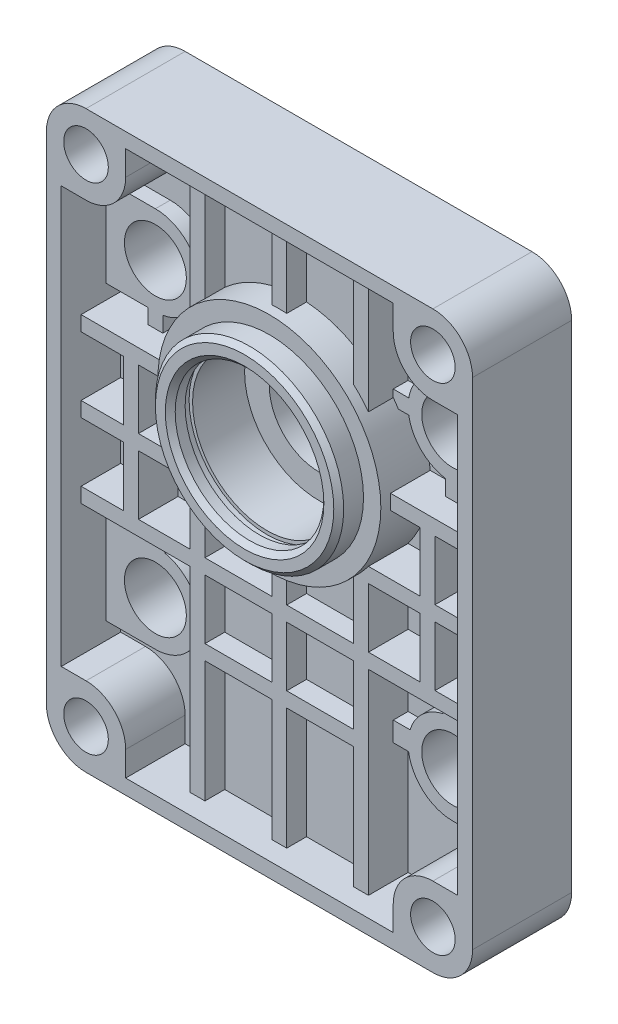
from build123d import *
from build123d.topology import SkipClean

# Parameters (mm, degrees)
EXTRUDE_1_DEPTH     = 12
SKETCH_2_R          = 22.5
EXTRUDE_2_DEPTH     = 6
SKETCH_3_R          = 19
EXTRUDE_3_DEPTH     = 5
EXTRUDE_4_DEPTH     = 8
SKETCH_5_W          = 10.424096596
SKETCH_5_H          = 12
SKETCH_5_W_2        = 13.5
EXTRUDE_5_DEPTH     = 4
CUT_EXTRUDE_START   = -4
SKETCH_6_W          = 8.575903404
SKETCH_6_H          = 12
SKETCH_6_W_2        = 10.424096596
CUT_EXTRUDE_1_DEPTH = 4
EXTRUDE_6_DEPTH     = 3
SKETCH_8_R          = 6.25
CUT_EXTRUDE_2_DEPTH = 87.423376467
SKETCH_9_R          = 4.5
CUT_EXTRUDE_3_DEPTH = 88.891979156
SKETCH_10_R         = 4
CUT_EXTRUDE_4_DEPTH = 6
CHAMFER_1_SIZE      = 1


with BuildPart() as part:
    # 草图1 → 凸台-拉伸1 (new body)
    with BuildSketch(Plane.XY):
        with BuildLine():
            Line((-43, 34), (-43, -66))
            ThreePointArc((-43, -66), (-40.656854249, -71.656854249), (-35, -74))
            Line((-35, -74), (35, -74))
            ThreePointArc((35, -74), (40.656854249, -71.656854249), (43, -66))
            Line((43, -66), (43, 34))
            ThreePointArc((43, 34), (40.656854249, 39.656854249), (35, 42))
            Line((35, 42), (-35, 42))
            ThreePointArc((-35, 42), (-40.656854249, 39.656854249), (-43, 34))
        make_face()
    extrude(amount=EXTRUDE_1_DEPTH)

    # 草图2 → 凸台-拉伸2 (add)
    with BuildSketch(Plane.XY.offset(12)):
        Circle(SKETCH_2_R)
    extrude(amount=EXTRUDE_2_DEPTH)

    # 草图3 → 凸台-拉伸3 (add)
    with BuildSketch(Plane.XY.offset(18)):
        Circle(SKETCH_3_R)
    extrude(amount=EXTRUDE_3_DEPTH)

    # 草图4 → 凸台-拉伸4 (add)
    with BuildSketch(Plane.XY.offset(12)):
        with BuildLine():
            Line((43, -66), (43, 34))
            ThreePointArc((43, 34), (40.656854249, 39.656854249), (35, 42))
            Line((35, 42), (-35, 42))
            ThreePointArc((-35, 42), (-40.656854249, 39.656854249), (-43, 34))
            Line((-43, 34), (-43, -66))
            ThreePointArc((-43, -66), (-40.656854249, -71.656854249), (-35, -74))
            Line((-35, -74), (35, -74))
            ThreePointArc((35, -74), (40.656854249, -71.656854249), (43, -66))
        make_face()
        with BuildLine():
            Line((35, -58), (40, -58))
            Line((40, -58), (40, 26))
            Line((40, 26), (35, 26))
            ThreePointArc((35, 26), (29.343145751, 28.343145751), (27, 34))
            Line((27, 34), (27, 39))
            Line((27, 39), (-27, 39))
            Line((-27, 39), (-27, 34))
            ThreePointArc((-27, 34), (-29.343145751, 28.343145751), (-35, 26))
            Line((-35, 26), (-40, 26))
            Line((-40, 26), (-40, -58))
            Line((-40, -58), (-35, -58))
            ThreePointArc((-35, -58), (-29.343145751, -60.343145751), (-27, -66))
            Line((-27, -66), (-27, -71))
            Line((-27, -71), (27, -71))
            Line((27, -71), (27, -66))
            ThreePointArc((27, -66), (29.343145751, -60.343145751), (35, -58))
        make_face(mode=Mode.SUBTRACT)
    extrude(amount=EXTRUDE_4_DEPTH)

    # 草图5 → 凸台-拉伸5 (add)
    # profile 1 of 3: a face of its own
    with BuildSketch(Plane.XY.offset(12)):
        with BuildLine():
            Line((-15, 16.770509831), (-15, 39))
            Line((-15, 39), (-18, 39))
            Line((-18, 39), (-18, 13.5))
            ThreePointArc((-18, 13.5), (-16.580834075, 15.209403057), (-15, 16.770509831))
        make_face()
    # profile 2 of 3: a face of its own
    with BuildSketch(Plane.XY.offset(12)):
        with BuildLine():
            Line((0, -71), (0, -22.5))
            ThreePointArc((0, -22.5), (-0.750417479, -22.487482598), (-1.5, -22.449944321))
            Line((-1.5, -22.449944321), (-1.5, -28.5))
            Line((-1.5, -28.5), (-15, -28.5))
            Line((-15, -28.5), (-15, -16.770509831))
            ThreePointArc((-15, -16.770509831), (-16.580834075, -15.209403057), (-18, -13.5))
            Line((-18, -13.5), (-28.424096596, -13.5))
            Line((-28.424096596, -13.5), (-28.424096596, -1.5))
            Line((-28.424096596, -1.5), (-22.449944321, -1.5))
            ThreePointArc((-22.449944321, -1.5), (-22.5, 0), (-22.449944321, 1.5))
            Line((-22.449944321, 1.5), (-40, 1.5))
            Line((-40, 1.5), (-40, -1.5))
            Line((-40, -1.5), (-31.424096596, -1.5))
            Line((-31.424096596, -1.5), (-31.424096596, -13.5))
            Line((-31.424096596, -13.5), (-40, -13.5))
            Line((-40, -13.5), (-40, -16.5))
            Line((-40, -16.5), (-31.424096596, -16.5))
            Line((-31.424096596, -16.5), (-31.424096596, -28.5))
            Line((-31.424096596, -28.5), (-40, -28.5))
            Line((-40, -28.5), (-40, -31.5))
            Line((-40, -31.5), (-18, -31.5))
            Line((-18, -31.5), (-18, -71))
            Line((-18, -71), (-15, -71))
            Line((-15, -71), (-15, -46.5))
            Line((-15, -46.5), (-1.5, -46.5))
            Line((-1.5, -46.5), (-1.5, -71))
            Line((-1.5, -71), (0, -71))
        make_face()
        with Locations((-23.212048298, -22.5)):
            Rectangle(SKETCH_5_W, SKETCH_5_H, mode=Mode.SUBTRACT)
        with Locations((-8.25, -37.5)):
            Rectangle(SKETCH_5_W_2, SKETCH_5_H, mode=Mode.SUBTRACT)
    # profile 3 of 3: a face of its own
    with BuildSketch(Plane.XY.offset(12)):
        with BuildLine():
            Line((0, 22.5), (0, 39))
            Line((0, 39), (-1.5, 39))
            Line((-1.5, 39), (-1.5, 22.449944321))
            ThreePointArc((-1.5, 22.449944321), (-0.750417479, 22.487482598), (0, 22.5))
        make_face()
    extrude_5 = extrude(amount=EXTRUDE_5_DEPTH)

    # 镜向1: 凸台-拉伸5 across plane
    add(extrude_5.mirror(Plane(origin=(0, 0, 0), x_dir=(0, 0, 1), z_dir=(1, 0, 0))))

    # 草图6 → 切除-拉伸1 (cut)
    with SkipClean():  # the faces are left unmerged after this step: merging them gives an invalid solid
        with BuildSketch(Plane.XY.offset(12).offset(CUT_EXTRUDE_START)):
            with Locations((-35.712048298, -7.5)):
                Rectangle(SKETCH_6_W, SKETCH_6_H)
            with BuildLine():
                Line((-28.424096596, -1.5), (-28.424096596, -13.5))
                Line((-28.424096596, -13.5), (-18, -13.5))
                ThreePointArc((-18, -13.5), (-21.096196313, -7.823074914), (-22.449944321, -1.5))
                Line((-22.449944321, -1.5), (-28.424096596, -1.5))
            make_face()
            with Locations((-35.712048298, -22.5)):
                Rectangle(SKETCH_6_W, SKETCH_6_H)
            with Locations((-23.212048298, -22.5)):
                Rectangle(SKETCH_6_W_2, SKETCH_6_H)
            with Locations((35.712048298, -7.5)):
                Rectangle(SKETCH_6_W, SKETCH_6_H)
            with Locations((35.712048298, -22.5)):
                Rectangle(SKETCH_6_W, SKETCH_6_H)
            with Locations((23.212048298, -22.5)):
                Rectangle(SKETCH_6_W_2, SKETCH_6_H)
            with BuildLine():
                Line((28.424096596, -1.5), (28.424096596, -13.5))
                Line((28.424096596, -13.5), (18, -13.5))
                ThreePointArc((18, -13.5), (21.096196313, -7.823074914), (22.449944321, -1.5))
                Line((22.449944321, -1.5), (28.424096596, -1.5))
            make_face()
            with BuildLine():
                Line((-40, 26), (-40, 1.5))
                Line((-40, 1.5), (-22.449944321, 1.5))
                ThreePointArc((-22.449944321, 1.5), (-21.096196313, 7.823074914), (-18, 13.5))
                Line((-18, 13.5), (-18, 39))
                Line((-18, 39), (-27, 39))
                Line((-27, 39), (-27, 34))
                ThreePointArc((-27, 34), (-29.343145751, 28.343145751), (-35, 26))
                Line((-35, 26), (-40, 26))
            make_face()
            with BuildLine():
                Line((18, 13.5), (18, 39))
                Line((18, 39), (27, 39))
                Line((27, 39), (27, 34))
                ThreePointArc((27, 34), (29.343145751, 28.343145751), (35, 26))
                Line((35, 26), (40, 26))
                Line((40, 26), (40, 1.5))
                Line((40, 1.5), (22.449944321, 1.5))
                ThreePointArc((22.449944321, 1.5), (21.096196313, 7.823074914), (18, 13.5))
            make_face()
            with BuildLine():
                Line((-40, -58), (-40, -31.5))
                Line((-40, -31.5), (-18, -31.5))
                Line((-18, -31.5), (-18, -71))
                Line((-18, -71), (-27, -71))
                Line((-27, -71), (-27, -66))
                ThreePointArc((-27, -66), (-29.343145751, -60.343145751), (-35, -58))
                Line((-35, -58), (-40, -58))
            make_face()
            with BuildLine():
                Line((40, -58), (40, -31.5))
                Line((40, -31.5), (18, -31.5))
                Line((18, -31.5), (18, -71))
                Line((18, -71), (27, -71))
                Line((27, -71), (27, -66))
                ThreePointArc((27, -66), (29.343145751, -60.343145751), (35, -58))
                Line((35, -58), (40, -58))
            make_face()
        extrude(amount=CUT_EXTRUDE_1_DEPTH, mode=Mode.SUBTRACT)

    # 草图7 → 凸台-拉伸6 (add)
    with SkipClean():  # the faces are left unmerged after this step: merging them gives an invalid solid
        with BuildSketch(Plane.XY.offset(8)):
            with BuildLine():
                Line((-30, 22.5), (-40, 22.5))
                Line((-40, 22.5), (-40, 4.5))
                Line((-40, 4.5), (-31.5, 4.5))
                Line((-31.5, 4.5), (-31.5, 1.5))
                Line((-31.5, 1.5), (-28.5, 1.5))
                Line((-28.5, 1.5), (-28.5, 4.625880325))
                ThreePointArc((-28.5, 4.625880325), (-23.636038969, 7.136038969), (-21.125880325, 12))
                Line((-21.125880325, 12), (-18, 12))
                Line((-18, 12), (-18, 15))
                Line((-18, 15), (-21.125880325, 15))
                ThreePointArc((-21.125880325, 15), (-24.190524981, 20.373863542), (-30, 22.5))
            make_face()
            with BuildLine():
                Line((-31.5, -31.5), (-28.023620394, -31.5))
                Line((-28.023620394, -31.5), (-28.023620394, -36.719685447))
                ThreePointArc((-28.023620394, -36.719685447), (-23.881575765, -38.899629944), (-21.394428301, -42.864827192))
                Line((-21.394428301, -42.864827192), (-18, -42.864827192))
                Line((-18, -42.864827192), (-18, -46.817586404))
                Line((-18, -46.817586404), (-21.096968715, -46.817586404))
                ThreePointArc((-21.096968715, -46.817586404), (-24.120300928, -52.313893074), (-30, -54.5))
                Line((-30, -54.5), (-40, -54.5))
                Line((-40, -54.5), (-40, -36.5))
                Line((-40, -36.5), (-31.5, -36.5))
                Line((-31.5, -36.5), (-31.5, -31.5))
            make_face()
        extrude_6 = extrude(amount=EXTRUDE_6_DEPTH)

    # 镜向2: 凸台-拉伸6 across plane
    with SkipClean():  # the faces are left unmerged after this step: merging them gives an invalid solid
        add(extrude_6.mirror(Plane(origin=(0, 0, 0), x_dir=(0, 0, 1), z_dir=(1, 0, 0))))

    # 草图8 → 切除-拉伸2 (cut, through all)
    with SkipClean():  # the faces are left unmerged after this step: merging them gives an invalid solid
        with BuildSketch(Plane.XY.offset(11)):
            with Locations((-30, 13.5)):
                Circle(SKETCH_8_R)
            with Locations((30, 13.5)):
                Circle(SKETCH_8_R)
            with Locations((-30, -45.5)):
                Circle(SKETCH_8_R)
            with Locations((30, -45.5)):
                Circle(SKETCH_8_R)
        extrude(amount=-CUT_EXTRUDE_2_DEPTH, mode=Mode.SUBTRACT)

    # 草图9 → 切除-拉伸3 (cut, through all)
    with SkipClean():  # the faces are left unmerged after this step: merging them gives an invalid solid
        with BuildSketch(Plane.XY.offset(20)):
            with Locations((-35, 34)):
                Circle(SKETCH_9_R)
            with Locations((35, 34)):
                Circle(SKETCH_9_R)
            with Locations((-35, -66)):
                Circle(SKETCH_9_R)
            with Locations((35, -66)):
                Circle(SKETCH_9_R)
        extrude(amount=-CUT_EXTRUDE_3_DEPTH, mode=Mode.SUBTRACT)

    # 草图10 → 切除-拉伸4 (cut)
    with SkipClean():  # the faces are left unmerged after this step: merging them gives an invalid solid
        with BuildSketch(Plane(origin=(0, 0, 0), x_dir=(-1, 0, 0), z_dir=(0, 0, -1))):
            with Locations((0, 31)):
                Circle(SKETCH_10_R)
            with Locations((0, -64)):
                Circle(SKETCH_10_R)
        extrude(amount=-CUT_EXTRUDE_4_DEPTH, mode=Mode.SUBTRACT)

    # 草图11 → 切除-旋转1 (revolve, cut)
    with SkipClean():  # the faces are left unmerged after this step: merging them gives an invalid solid
        with BuildSketch(Plane(origin=(0, 0, 0), x_dir=(0, 0, -1), z_dir=(1, 0, 0)), mode=Mode.PRIVATE) as cut_revolve_1_sk:
            Polygon((0, 0), (0, 10), (-8, 10), (-8, 15), (-18.5, 15), (-18.5, 15.7), (-20, 15.7), (-20, 15), (-23, 15), (-23, 0), align=None)
        revolve(cut_revolve_1_sk.sketch.rotate(Axis((0, 0, -10.866098112), (0, 0, 1)), 90), axis=Axis((0, 0, -10.866098112), (0, 0, 1)), mode=Mode.SUBTRACT)

    # 倒角1
    chamfer_1_edges = [part.edges().sort_by_distance(p)[0] for p in [
        (-19, 0, 23),
        (15, 0, 23),
    ]]
    chamfer(chamfer_1_edges, length=CHAMFER_1_SIZE)


solid = part.part
